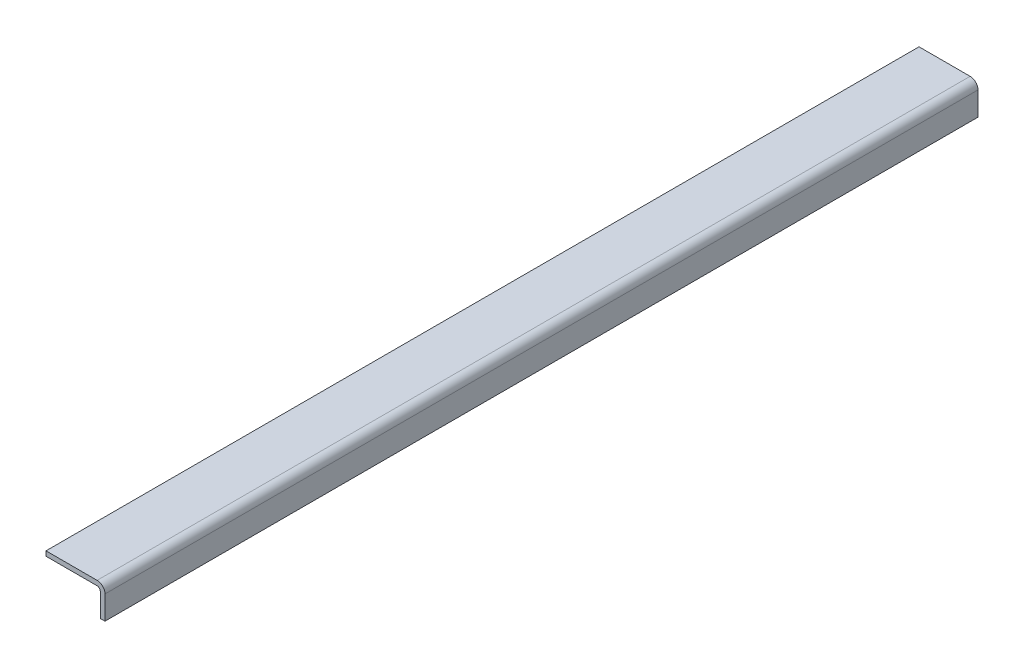
from build123d import *

# Parameters (mm, degrees)
BOSS_EXTRUDE1_DEPTH = 1110


with BuildPart() as part:
    # Sketch1 → Boss-Extrude1 (new body)
    with BuildSketch(Plane.XY):
        with BuildLine():
            Line((0, 0), (65, 0))
            ThreePointArc((65, 0), (72.071067812, -2.928932188), (75, -10))
            Line((75, -10), (75, -40))
            Line((75, -40), (69, -40))
            Line((69, -40), (69, -10))
            ThreePointArc((69, -10), (67.828427125, -7.171572875), (65, -6))
            Line((65, -6), (0, -6))
            Line((0, -6), (0, 0))
        make_face()
    extrude(amount=BOSS_EXTRUDE1_DEPTH)


solid = part.part
